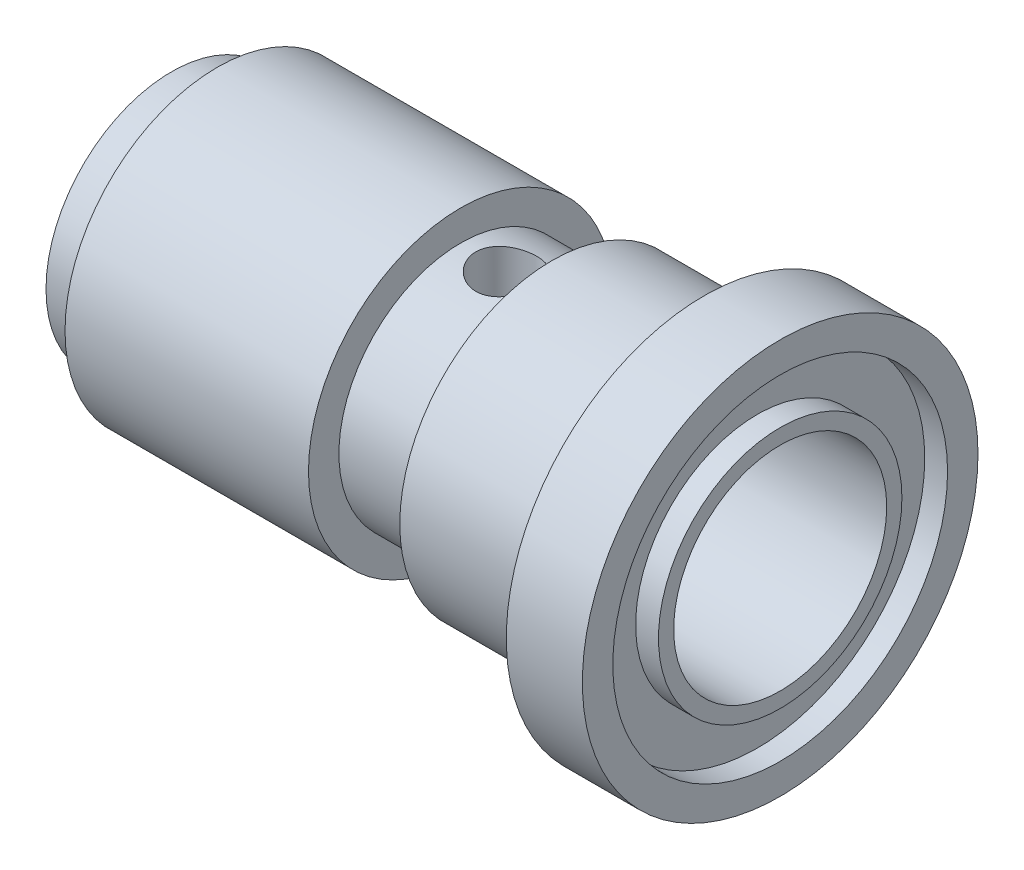
from build123d import *

# Parameters (mm, degrees)
SKETCH1_R            = 8.25
BOSS_EXTRUDE1_DEPTH  = 3
SKETCH2_R            = 10
BOSS_EXTRUDE2_DEPTH  = 32
SKETCH4_R            = 13
BOSS_EXTRUDE3_DEPTH  = 5
SKETCH5_R            = 7
CUT_EXTRUDE1_DEPTH   = 10
SKETCH6_R            = 2.5
CUT_EXTRUDE2_DEPTH   = 33
SKETCH7_R            = 3.75
CUT_EXTRUDE3_DEPTH   = 6.5
CUT_SWEEP1_PROFILE_R = 2
SKETCH15_W           = 6
SKETCH15_H           = 4.8134745
CUT_EXTRUDE4_START   = -1.5
SKETCH17_R           = 11
SKETCH17_R_2         = 8
CUT_EXTRUDE4_DEPTH   = 1.5


with BuildPart() as part:
    # Sketch1 → Boss-Extrude1 (new body)
    with BuildSketch(Plane(origin=(0, 0, 0), x_dir=(0, 0, -1), z_dir=(1, 0, 0))):
        Circle(SKETCH1_R)
    extrude(amount=BOSS_EXTRUDE1_DEPTH)

    # Sketch2 → Boss-Extrude2 (add)
    with BuildSketch(Plane(origin=(3, 0, 0), x_dir=(0, 0, -1), z_dir=(1, 0, 0))):
        Circle(SKETCH2_R)
    extrude(amount=BOSS_EXTRUDE2_DEPTH)

    # Sketch4 → Boss-Extrude3 (add)
    with BuildSketch(Plane(origin=(35, 0, 0), x_dir=(0, 0, -1), z_dir=(1, 0, 0))):
        Circle(SKETCH4_R)
    extrude(amount=BOSS_EXTRUDE3_DEPTH)

    # Sketch5 → Cut-Extrude1 (cut)
    with BuildSketch(Plane(origin=(40, 0, 0), x_dir=(0, 0, -1), z_dir=(1, 0, 0))):
        Circle(SKETCH5_R)
    extrude(amount=-CUT_EXTRUDE1_DEPTH, mode=Mode.SUBTRACT)

    # Sketch6 → Cut-Extrude2 (cut)
    with BuildSketch(Plane(origin=(30, 0, 0), x_dir=(0, 0, -1), z_dir=(1, 0, 0))):
        Circle(SKETCH6_R)
    extrude(amount=-CUT_EXTRUDE2_DEPTH, mode=Mode.SUBTRACT)

    # Sketch7 → Cut-Extrude3 (cut)
    with BuildSketch(Plane.ZY):
        Circle(SKETCH7_R)
    extrude(amount=-CUT_EXTRUDE3_DEPTH, mode=Mode.SUBTRACT)

    # Cut-Sweep1: sweep along a path in Sketch8
    with BuildLine(Plane.XY) as cut_sweep1_path:
        Line((22, 11.268162534), (22, -10.569361757))
    # Cut-Sweep1 profile (on start of the path) → Cut-Sweep1 (sweep, cut)
    with BuildSketch(Plane(origin=(22, 11.268162534, 0), x_dir=(-1, 0, 0), z_dir=(0, -1, 0))):
        Circle(CUT_SWEEP1_PROFILE_R)
    sweep(path=cut_sweep1_path.line, mode=Mode.SUBTRACT)

    # Sketch15 → Cut-Revolve1 (revolve, cut)
    with BuildSketch(Plane.XY, mode=Mode.PRIVATE) as cut_revolve1_sk:
        with Locations((22, 10.40673725)):
            Rectangle(SKETCH15_W, SKETCH15_H)
    revolve(cut_revolve1_sk.sketch.rotate(Axis((0, 0, 0), (-1, 0, 0)), 90), axis=Axis((0, 0, 0), (-1, 0, 0)), mode=Mode.SUBTRACT)

    # Sketch17 → Cut-Extrude4 (cut)
    with BuildSketch(Plane(origin=(40, 0, 0), x_dir=(0, 0, -1), z_dir=(1, 0, 0)).offset(CUT_EXTRUDE4_START)):
        Circle(SKETCH17_R)
        Circle(SKETCH17_R_2, mode=Mode.SUBTRACT)
    extrude(amount=CUT_EXTRUDE4_DEPTH, mode=Mode.SUBTRACT)


solid = part.part
